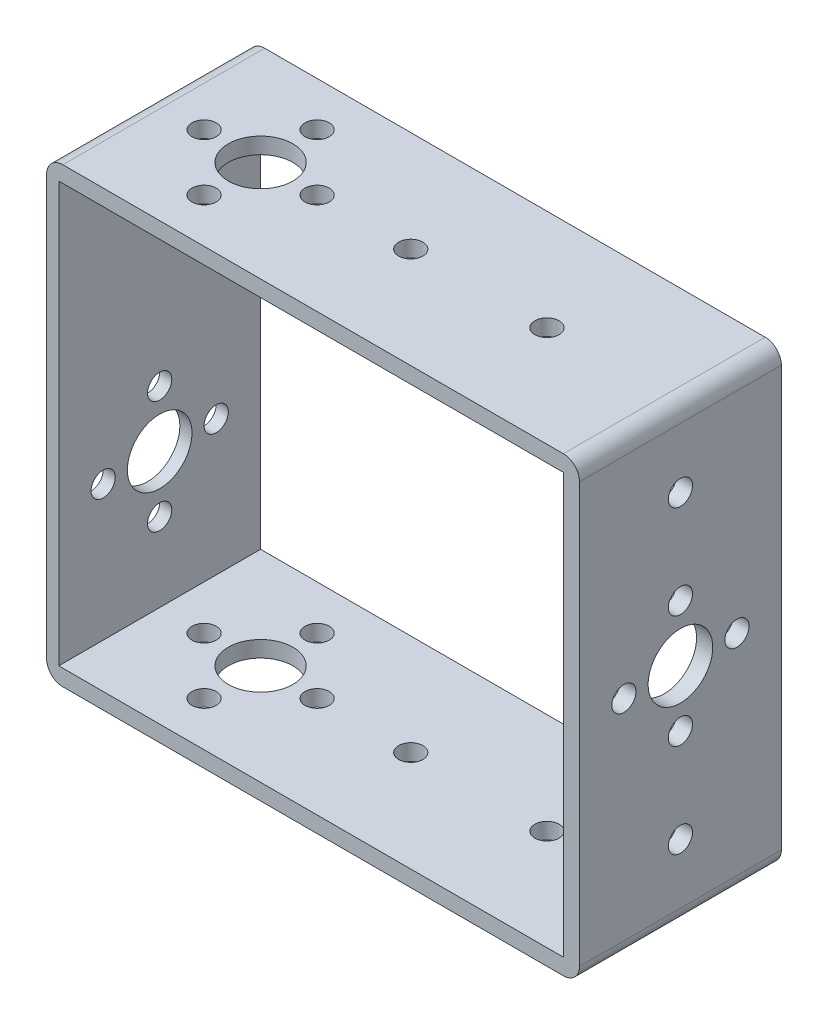
SolidWorks part; units mm, degrees
ref_plane "Front Plane" through (0, 0, 0) normal (0, 0, 1) x (1, 0, 0)
ref_plane "Top Plane" through (0, 0, 0) normal (0, 1, 0) x (1, 0, 0)
ref_plane "Right Plane" through (0, 0, 0) normal (1, 0, 0) x (0, 0, -1)
other "Configuration Table"
sketch "Sketch1" plane through (0, 0, 0) normal (0, 0, 1) x (1, 0, 0)
  line L1 (-32.25, 28) -> (32.25, 28)
  line L2 (-32.25, 28) -> (-32.25, -28)
  line L3 (-32.25, -28) -> (32.25, -28)
  line L4 (32.25, 28) -> (32.25, -28)
  line L5 (-32.25, 28) -> (32.25, -28) construction
  line L6 (-32.25, -28) -> (32.25, 28) construction
  point P0 (0, 0)
  dimension "D1" = 64.5
  dimension "D2" = 56
extrude "Boss-Extrude1" add sketch "Sketch1" along normal blind 25
sketch "Sketch2" plane through (0, 0, 25) normal (0, 0, 1) x (1, 0, 0)
  line L0 (-32.25, 28) -> (-32.25, -28) construction
  line L1 (-32.25, 26) -> (30.25, 26)
  line L2 (-32.25, 26) -> (-32.25, -26)
  line L3 (-32.25, -26) -> (30.25, -26)
  line L4 (30.25, 26) -> (30.25, -26)
  line L5 (-32.25, -28) -> (32.25, -28) construction
  line L6 (32.25, 28) -> (-32.25, 28) construction
  line L7 (32.25, -28) -> (32.25, 28) construction
  dimension "D1" = 2
  dimension "D2" = 2
  dimension "D3" = 2
extrude "Cut-Extrude1" cut sketch "Sketch2" against normal up to next
sketch "Sketch3" plane through (32.25, 0, 0) normal (1, 0, 0) x (0, 0, -1)
  line L0 (0, 0) -> (-43.1082, 0) construction
  line L1 (0, 0) -> (0, -32.0286) construction
  line L2 (-25, -28) -> (-25, 28) construction
  circle A0 centre (-12.5, 0) radius 4
  circle A1 centre (-12.5, 0) radius 7 construction
  circle A2 centre (-5.5, 0) radius 1.5
  circle A3 centre (-12.5, 18.6) radius 1.5
  circle A4 centre (-12.5, -7) radius 1.5
  circle A5 centre (-19.5, 0) radius 1.5
  circle A6 centre (-12.5, 7) radius 1.5
  circle A7 centre (-12.5, -18.6) radius 1.5
  point P22 (-12.5, 0)
  dimension "D1" = 8
  dimension "D2" = 14
  dimension "D3" = 3
  dimension "D4" = 3
  dimension "D5" = 18.6
  dimension "D6" = 12.5
  dimension "D7" = 12.5
  dimension "D8" = 4
extrude "Cut-Extrude2" cut sketch "Sketch3" against normal up to next
sketch "Sketch4" plane through (0, -28, 0) normal (0, -1, 0) x (1, 0, 0)
  line L0 (-36.174, 12.5) -> (44.1516, 12.5) construction
  line L1 (0, 0) -> (0, 35.8464) construction
  line L2 (-32.25, 25) -> (32.25, 25) construction
  line L3 (-32.25, 25) -> (-32.25, 0) construction
  line L4 (-19.75, 12.5) -> (-19.75, -11.9582) construction
  circle A0 centre (-19.75, 12.5) radius 4
  circle A1 centre (-19.75, 12.5) radius 7 construction
  circle A2 centre (-12.75, 12.5) radius 1.5
  circle A3 centre (-1.15, 12.5) radius 1.5
  circle A4 centre (15.72, 12.5) radius 1.5
  circle A5 centre (-19.75, 5.5) radius 1.5
  circle A6 centre (-26.75, 12.5) radius 1.5
  circle A7 centre (-19.75, 19.5) radius 1.5
  point P25 (-19.75, 12.5)
  dimension "D2" = 8
  dimension "D3" = 14
  dimension "D4" = 3
  dimension "D5" = 3
  dimension "D6" = 3
  dimension "D1" = 12.5
  dimension "D7" = 16.87
  dimension "D9" = 50
  dimension "D10" = 18.6
  dimension "D11" = 12.5
  dimension "D8" = 4
extrude "Cut-Extrude3" cut sketch "Sketch4" against normal up to next
mirror "Mirror1" about plane through (0, 0, 0) normal (0, 1, 0) of "Cut-Extrude3"
fillet "Fillet3" radius 2 2 edges at (32.25, -28, 12.5) (32.25, 28, 12.5)
sketch "Sketch5" plane through (0, 0, 0) normal (0, 1, 0) x (1, 0, 0)
  line L0 (30.25, -25) -> (-32.25, -25) construction
  line L1 (-32.25, 0) -> (-33.75, 0)
  line L2 (-32.25, 0) -> (-32.25, -25)
  line L3 (-32.25, -25) -> (-33.75, -25)
  line L4 (-33.75, 0) -> (-33.75, -25)
  dimension "D1" = 1.5
extrude "Boss-Extrude2" add sketch "Sketch5" along normal up to surface and the other way up to surface up to face at (-19.75, 28, 4) other way up to face at (-19.75, -28, 4)
fillet "Fillet4" radius 2 2 edges at (-33.75, 28, 12.5) (-33.75, -28, 12.5)
sketch "Sketch6" plane through (-32.25, 0, 0) normal (1, 0, 0) x (0, 0, -1)
  line L0 (-12.5, -26) -> (-12.5, 30.7922) construction
  line L1 (0, -26) -> (-25, -26) construction
  line L2 (-25, -28) -> (0, -28) construction
  line L3 (-12.5, -9.25) -> (-0.5354, -9.25) construction
  circle A0 centre (-12.5, -9.25) radius 4
  circle A1 centre (-12.5, -9.25) radius 7 construction
  circle A2 centre (-12.5, -2.25) radius 1.5
  circle A3 centre (-5.5, -9.25) radius 1.5
  circle A4 centre (-12.5, -16.25) radius 1.5
  circle A5 centre (-19.5, -9.25) radius 1.5
  point P20 (-12.5, -9.25)
  dimension "D1" = 8
  dimension "D2" = 14
  dimension "D4" = 3
  dimension "D3" = 18.75
  dimension "D5" = 4
extrude "Cut-Extrude5" cut sketch "Sketch6" against normal up to surface (1.5 mm away) contours A2 | A5 | A3 | A4 | A0 up to face at (-33.75, 0, 12.5)
